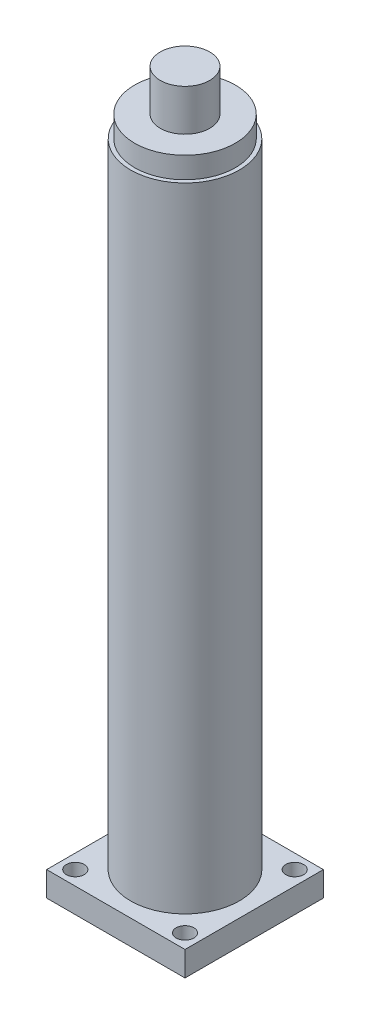
SolidWorks part; units mm, degrees
material "Q235B"
ref_plane "Front Plane" through (0, 0, 0) normal (0, 0, 1) x (1, 0, 0)
ref_plane "Top Plane" through (0, 0, 0) normal (0, 1, 0) x (1, 0, 0)
ref_plane "Right Plane" through (0, 0, 0) normal (1, 0, 0) x (0, 0, -1)
sketch "Sketch1" plane through (0, 0, 0) normal (0, 0, 1) x (1, 0, 0)
  line L0 (0, 0) -> (60, 0)
  line L1 (60, 0) -> (60, 25)
  line L2 (60, 25) -> (55, 25)
  line L3 (55, 25) -> (55, 665.5)
  line L4 (55, 665.5) -> (51, 665.5)
  line L5 (51, 665.5) -> (51, 687)
  line L6 (51, 687) -> (25, 687)
  line L7 (25, 687) -> (25, 729)
  line L8 (25, 729) -> (0, 729)
  line L9 (0, 729) -> (0, 0)
  line L10 (0, 0) -> (0, -53.7521) construction
  dimension "D1" = 120
  dimension "D2" = 110
  dimension "D3" = 102
  dimension "D4" = 50
  dimension "D5" = 25
  dimension "D6" = 42
  dimension "D7" = 21.5
  dimension "D8" = 729
revolve "Revolve1" add sketch "Sketch1" angle 360 about L10
sketch "Sketch2" plane through (0, 0, 0) normal (0, 1, 0) x (1, 0, 0)
  line L1 (70, -70) -> (-70, -70)
  line L2 (70, -70) -> (70, 70)
  line L3 (70, 70) -> (-70, 70)
  line L4 (-70, -70) -> (-70, 70)
  line L5 (70, -70) -> (-70, 70) construction
  line L6 (70, 70) -> (-70, -70) construction
  circle A0 centre (-55.5, 55.5) radius 9
  circle A1 centre (55.5, 55.5) radius 9
  circle A2 centre (55.5, -55.5) radius 9
  circle A3 centre (-55.5, -55.5) radius 9
  point P0 (0, 0)
  point P17 (0, 0)
  dimension "D2" = 18
  dimension "D4" = 111
  dimension "D1" = 140
  dimension "D3" = 4
extrude "Boss-Extrude1" add sketch "Sketch2" along normal blind 25
